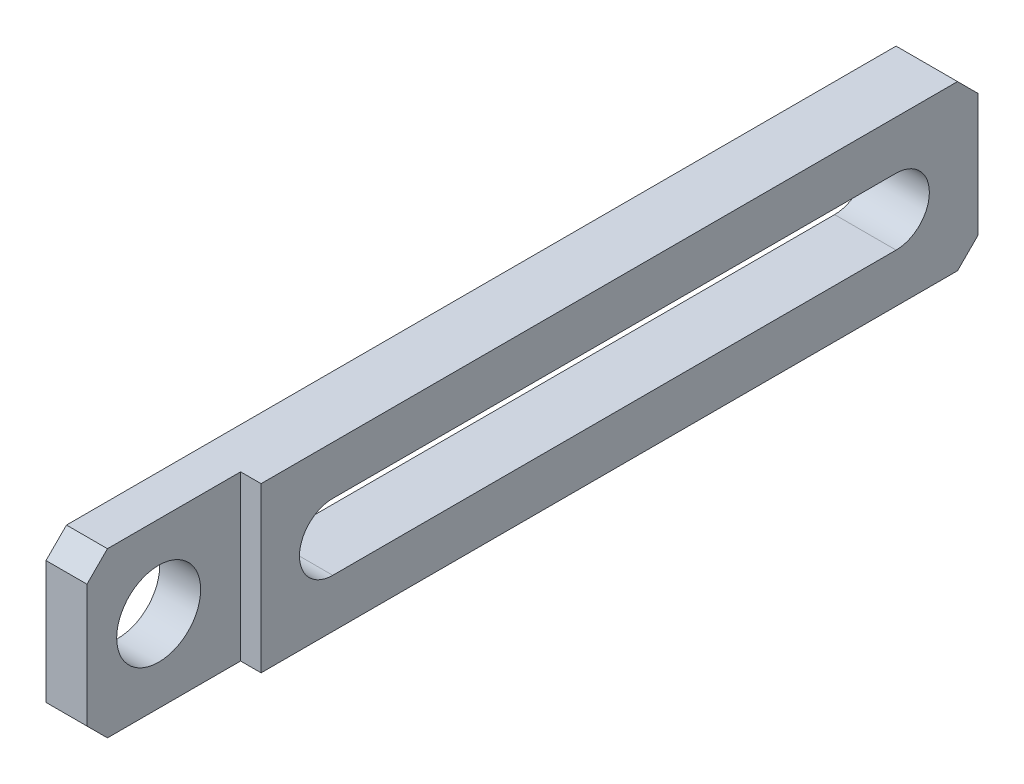
SolidWorks part; units mm, degrees
material "6061-T6"
ref_plane "Front Plane" through (0, 0, 0) normal (0, 0, 1) x (1, 0, 0)
ref_plane "Top Plane" through (0, 0, 0) normal (0, 1, 0) x (1, 0, 0)
ref_plane "Right Plane" through (0, 0, 0) normal (1, 0, 0) x (0, 0, -1)
sketch "Sketch1" plane through (0, 0, 0) normal (1, 0, 0) x (0, 0, -1)
  line L0 (22, -4.75) -> (77, -4.75)
  line L1 (0, 0) -> (85, 0)
  line L2 (0, 0) -> (0, -16)
  line L3 (0, -16) -> (85, -16)
  line L4 (85, 0) -> (85, -16)
  line L5 (22, -11.25) -> (77, -11.25)
  arc A0 (77, -11.25) -> (77, -4.75) centre (77, -8) ccw
  arc A1 (22, -4.75) -> (22, -11.25) centre (22, -8) ccw
  dimension "D6" = 6.5
  dimension "D1" = 85
  dimension "D2" = 16
  dimension "D3" = 8
  dimension "D4" = 8
  dimension "D5" = 55
extrude "Extrude1" add sketch "Sketch1" along normal blind 6
hole_wizard "Ø8.2 (8.2) Diameter Hole1" positions "Sketch4" profile "Sketch3" hole size "Ø8.2" standard "ISO" end condition through all
sketch "Sketch4" plane through (6, 0, 0) normal (1, 0, 0) x (0, 0, -1)
  line L1 (0, -16) -> (85, -16) construction
  line L2 (0, 0) -> (0, -16) construction
  point P0 (7, -8)
  dimension "D1" = 7
  dimension "D2" = 8
sketch "Sketch3" plane through (6, -8, -7) normal (0, 1, 0) x (0, 0, -1)
  line L0 (0, 0) -> (0, 6)
  line L1 (0, 6) -> (4.1, 6)
  line L2 (4.1, 6) -> (4.1, 0)
  line L5 (4.1, 0) -> (0, 0)
  line L11 (0, -6.35) -> (0, 107.95) construction
  dimension "通孔孔直径" = 8.2
  dimension "通孔孔深度" = 6
chamfer "Chamfer1" distance 2 angle 45 4 edges at (3, 0, -85) (3, -16, -85) (3, -16, 0) (3, 0, 0)
sketch "Sketch5" plane through (6, 0, 0) normal (1, 0, 0) x (0, 0, -1)
  line L0 (83, 0) -> (2, 0) construction
  line L1 (15, 0) -> (0, 0)
  line L2 (15, 0) -> (15, -16)
  line L3 (15, -16) -> (0, -16)
  line L4 (0, 0) -> (0, -16)
  line L5 (2, -16) -> (83, -16) construction
  line L6 (0, -2) -> (0, -14) construction
  dimension "D1" = 15
extrude "Cut-Extrude1" cut sketch "Sketch5" against normal blind 2
